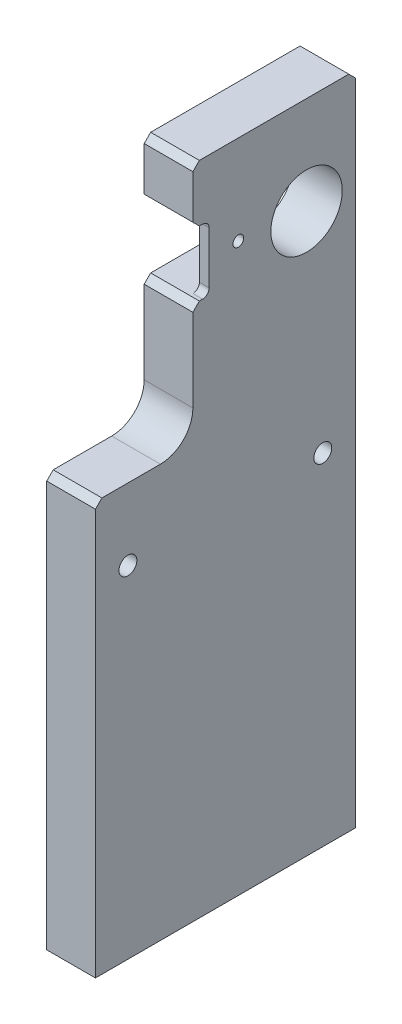
SolidWorks part; units mm, degrees
material "A6061"
ref_plane "前基準面" through (0, 0, 0) normal (0, 0, 1) x (1, 0, 0)
ref_plane "上基準面" through (0, 0, 0) normal (0, 1, 0) x (1, 0, 0)
ref_plane "右基準面" through (0, 0, 0) normal (1, 0, 0) x (0, 0, -1)
sketch "草图1" plane through (0, 0, 0) normal (1, 0, 0) x (0, 0, -1)
  line L0 (-10, 101) -> (-10, 36)
  line L1 (-10, 101) -> (40, 101)
  line L2 (-40, 26) -> (-40, -101)
  line L3 (-40, -101) -> (40, -101)
  line L4 (40, 101) -> (40, -101)
  line L5 (-40, 101) -> (40, -101) construction
  line L6 (-40, -101) -> (40, 101) construction
  line L7 (-20, 26) -> (-40, 26)
  arc A0 (-10, 36) -> (-20, 26) centre (-20, 36) cw
  point P0 (0, 0)
  dimension "D4" = 10
  dimension "D1" = 202
  dimension "D2" = 80
  dimension "D3" = 75
  dimension "D5" = 30
extrude "凸台-拉伸1" add sketch "草图1" along normal mid plane 15
sketch "草图2" plane through (-7.5, 0, 0) normal (-1, 0, 0) x (0, 0, 1)
  line L0 (-40, -101) -> (-40, 101) construction
  line L2 (-40, 101) -> (10, 101) construction
  circle A0 centre (-25, 71) radius 11
  dimension "D1" = 22
  dimension "D2" = 15
  dimension "D3" = 30
extrude "切除-拉伸1" cut sketch "草图2" against normal through all
hole_wizard "M5 螺纹孔1" positions "草图6" profile "草图7" tap size "M5" standard "GB"
sketch "草图6" plane through (0, -101, 0) normal (0, -1, 0) x (-1, 0, 0)
  line L0 (-7.5, 0) -> (7.5, 0) construction
  line L1 (-7.5, -40) -> (-7.5, 40) construction
  line L3 (7.5, -40) -> (7.5, 40) construction
  point P0 (0, 25)
  point P9 (0, -25)
  dimension "D1" = 50
sketch "草图7" plane through (0, -101, -25) normal (1, 0, 0) x (0, 0, -1)
  line L0 (0, 0) -> (0, 13.6618)
  line L1 (0, 13.6618) -> (2.1, 12.4)
  line L2 (2.1, 12.4) -> (2.1, 0)
  line L5 (2.1, 0) -> (0, 0)
  line L10 (0, 13.6618) -> (-2.1, 12.4) construction
  line L11 (0, -6.35) -> (0, 107.95) construction
  dimension "螺纹孔钻头直径" = 4.2
  dimension "螺纹孔钻头深度" = 12.4
  dimension "导头角度" = 118
cosmetic thread "孔螺蚊线3" parameters "D1"=10, "D2"=5
cosmetic thread "孔螺蚊线4" parameters "D1"=10, "D2"=5
hole_wizard "M5 六角圆柱头螺钉的柱形沉头孔1" positions "草图8" profile "草图9" counterbore size "M5" standard "GB" end condition through all
sketch "草图8" plane through (-7.5, 0, 0) normal (-1, 0, 0) x (0, 0, 1)
  line L0 (0, 0) -> (0, 35.1182) construction
  line L2 (40, -101) -> (-40, -101) construction
  point P0 (-30, 4)
  point P2 (30, 4)
  dimension "D1" = 60
  dimension "D2" = 105
sketch "草图9" plane through (-7.5, 4, -30) normal (0, 1, 0) x (0, 0, 1)
  line L0 (0, 0) -> (0, 15)
  line L1 (0, 15) -> (2.75, 15)
  line L3 (2.75, 15) -> (2.75, 5.7)
  line L4 (2.75, 5.7) -> (5, 5.7)
  line L5 (5, 5.7) -> (5, 0)
  line L7 (5, 0) -> (0, 0)
  line L11 (0, -6.35) -> (0, 107.95) construction
  dimension "通孔孔直径" = 5.5
  dimension "通孔孔深度" = 15
  dimension "柱形沉头孔直径" = 10
  dimension "柱形沉头孔深度" = 5.7
hole_wizard "M6 螺纹孔1" positions "草图10" profile "草图11" tap size "M6" standard "GB"
sketch "草图10" plane through (0, 0, -40) normal (0, 0, -1) x (-1, 0, 0)
  line L0 (0, 101) -> (0, 33.1066) construction
  line L1 (-7.5, 101) -> (7.5, 101) construction
  point P0 (0, 51)
  point P7 (0, 91)
  dimension "D1" = 40
  dimension "D2" = 10
sketch "草图11" plane through (0, 51, -40) normal (1, 0, 0) x (0, 1, 0)
  line L0 (0, 0) -> (0, 16.5022)
  line L1 (0, 16.5022) -> (2.5, 15)
  line L2 (2.5, 15) -> (2.5, 0)
  line L5 (2.5, 0) -> (0, 0)
  line L10 (0, 16.5022) -> (-2.5, 15) construction
  line L11 (0, -6.35) -> (0, 107.95) construction
  dimension "螺纹孔钻头直径" = 5
  dimension "螺纹孔钻头深度" = 15
  dimension "导头角度" = 118
cosmetic thread "孔螺蚊线5" parameters "D1"=12, "D2"=6
cosmetic thread "孔螺蚊线6" parameters "D1"=12, "D2"=6
chamfer "倒角1" distance 2 angle 45 3 edges at (0, 101, -40) (0, 26, 40) (0, 101, 10)
sketch "草图19" plane through (-7.5, 0, 0) normal (-1, 0, 0) x (0, 0, 1)
  line L0 (10, 99) -> (10, 36) construction
  line L1 (10, 80.5) -> (17, 80.5)
  line L2 (10, 80.5) -> (10, 66.5)
  line L3 (10, 66.5) -> (17, 66.5)
  line L4 (17, 80.5) -> (17, 66.5)
  line L6 (17, 73.5) -> (10, 73.5) construction
  line L7 (-38, 101) -> (8, 101) construction
  dimension "D1" = 14
  dimension "D2" = 7
  dimension "D3" = 27.5
extrude "凸台-拉伸2" [suppressed] add sketch "草图19" against normal up to surface (15 mm away)
sketch "草图20" plane through (-7.5, 0, 0) normal (-1, 0, 0) x (0, 0, 1)
  line L5 (-38, 101) -> (8, 101) construction
  line L6 (-40, -101) -> (-40, 99) construction
  circle A0 centre (11, 73.5) radius 15
  dimension "D1" = 30
  dimension "D2" = 27.5
  dimension "D3" = 51
extrude "切除-拉伸6" [suppressed] cut sketch "草图20" against normal offset from surface (7 mm away) 8
fillet "圆角1" [suppressed] radius 3
sketch "草图12" plane through (7.5, 0, 0) normal (1, 0, 0) x (0, 0, -1)
  line L0 (40, -101) -> (40, 99) construction
  line L1 (-40, -101) -> (40, -101) construction
  circle A0 centre (-11, 73.5) radius 2.5
  dimension "D1" = 5
  dimension "D3" = 174.5
  dimension "D2" = 51
extrude "切除-拉伸2" cut sketch "草图12" against normal through all
sketch "草图13" plane through (-7.5, 0, 0) normal (-1, 0, 0) x (0, 0, 1)
  line L0 (-40, -101) -> (-40, 99) construction
  line L1 (40, -101) -> (-40, -101) construction
  point P0 (-4, 73.5)
  dimension "D1" = 36
  dimension "D2" = 174.5
hole_wizard "M4 螺纹孔1" positions "草图13" profile "草图14" tap size "M4" standard "GB" end condition through all
sketch "草图14" plane through (-7.5, 73.5, -4) normal (0, 1, 0) x (0, 0, 1)
  line L0 (0, 0) -> (0, 15)
  line L1 (0, 15) -> (1.65, 15)
  line L2 (1.65, 15) -> (1.65, 0)
  line L5 (1.65, 0) -> (0, 0)
  line L11 (0, -6.35) -> (0, 107.95) construction
  dimension "通孔螺纹孔钻头直径" = 3.3
  dimension "通孔螺纹孔钻头深度" = 15
cosmetic thread "孔螺蚊线7" parameters "D2"=4
sketch "草图15" plane through (-7.5, 0, 0) normal (-1, 0, 0) x (0, 0, 1)
  line L0 (11, 73.5) -> (-32.6277, 73.5) construction
  line L1 (10, 99) -> (10, 75.7913) construction
  line L2 (-12, 63.5) -> (10, 63.5)
  line L3 (-12, 63.5) -> (-12, 83.5)
  line L4 (-12, 83.5) -> (10, 83.5)
  line L5 (10, 63.5) -> (10, 83.5)
  line L6 (-12, 63.5) -> (10, 83.5) construction
  line L7 (-12, 83.5) -> (10, 63.5) construction
  point P3 (-1, 73.5)
  dimension "D1" = 20
  dimension "D2" = 22
extrude "切除-拉伸3" cut sketch "草图15" against normal offset from surface (12 mm away) 3 up to face at (7.5, 73.5, -2.35)
sketch "草图16" plane through (4.5, 0, 0) normal (-1, 0, 0) x (0, 0, 1)
  line L1 (10, 83.5) -> (5, 83.5)
  line L2 (10, 83.5) -> (10, 63.5)
  line L3 (10, 63.5) -> (5, 63.5)
  line L4 (5, 83.5) -> (5, 63.5)
  line L5 (-12, 63.5) -> (10, 63.5) construction
  dimension "D1" = 20
  dimension "D2" = 5
extrude "切除-拉伸4" cut sketch "草图16" against normal through all
sketch "草图17" plane through (-7.5, 0, 0) normal (-1, 0, 0) x (0, 0, 1)
  circle A0 centre (-12, 83.5) radius 1
  circle A1 centre (-12, 63.5) radius 1
  dimension "D1" = 2
  dimension "D2" = 2
extrude "切除-拉伸5" cut sketch "草图17" against normal up to surface (12 mm away) up to face at (4.5, 73.5, -3.5)
chamfer "倒角2" distance 2 angle 45 2 edges at (0, 63.5, 10) (0, 83.5, 10)
fillet "圆角2" radius 2 2 edges at (6, 83.5, 5) (6, 63.5, 5)
